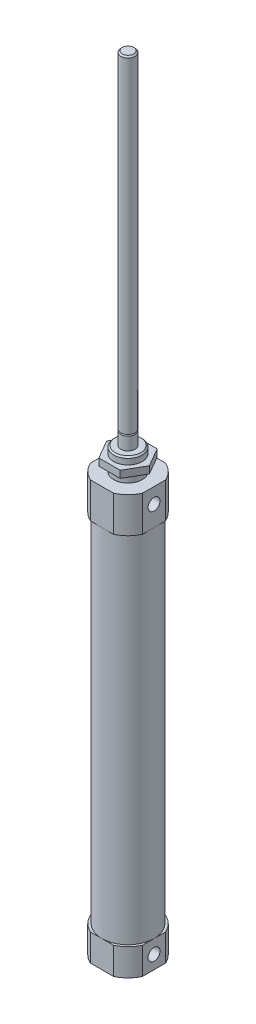
SolidWorks part; units mm, degrees
ref_plane "Front Plane" through (0, 0, 0) normal (0, 0, 1) x (1, 0, 0)
ref_plane "Top Plane" through (0, 0, 0) normal (0, 1, 0) x (1, 0, 0)
ref_plane "Right Plane" through (0, 0, 0) normal (1, 0, 0) x (0, 0, -1)
sketch "Sketch1" plane through (0, 0, 0) normal (0, 1, 0) x (1, 0, 0)
  line L0 (0, 0) -> (0, -50000) construction
  line L1 (-4.0345, 9.15) -> (4.0345, 9.15)
  line L2 (-9.15, 4.0345) -> (-9.15, -4.0345)
  line L3 (-4.0345, -9.15) -> (4.0345, -9.15)
  line L4 (9.15, 4.0345) -> (9.15, -4.0345)
  line L5 (0, 0) -> (50000, 0) construction
  arc A0 (4.0345, -9.15) -> (9.15, -4.0345) centre (0, 0) ccw
  arc A1 (9.15, 4.0345) -> (4.0345, 9.15) centre (0, 0) ccw
  arc A2 (-4.0345, 9.15) -> (-9.15, 4.0345) centre (0, 0) ccw
  arc A3 (-9.15, -4.0345) -> (-4.0345, -9.15) centre (0, 0) ccw
  point P0 (0, 0)
  dimension "D3" = 10
  dimension "D1" = 18.3
  dimension "D2" = 18.3
extrude "Boss-Extrude1" add sketch "Sketch1" along normal blind 12.5
sketch "Sketch3" plane through (0, 0, 0) normal (0, -1, 0) x (1, 0, 0)
  circle A0 centre (0, 0) radius 9.15
  dimension "D1" = 18.3
extrude "Boss-Extrude2" add sketch "Sketch3" along normal blind 125
sketch "Sketch4" plane through (0, -125, 0) normal (0, -1, 0) x (1, 0, 0)
  line L4 (-4.0345, 9.15) -> (4.0345, 9.15)
  line L5 (-9.15, -4.0345) -> (-9.15, 4.0345)
  line L6 (4.0345, -9.15) -> (-4.0345, -9.15)
  line L7 (9.15, 4.0345) -> (9.15, -4.0345)
  arc A4 (-4.0345, 9.15) -> (-9.15, 4.0345) centre (0, 0) ccw
  arc A5 (-9.15, -4.0345) -> (-4.0345, -9.15) centre (0, 0) ccw
  arc A6 (4.0345, -9.15) -> (9.15, -4.0345) centre (0, 0) ccw
  arc A7 (9.15, 4.0345) -> (4.0345, 9.15) centre (0, 0) ccw
extrude "Boss-Extrude3" add sketch "Sketch4" along normal blind 9.5
sketch "Sketch5" plane through (0, 12.5, 0) normal (0, 1, 0) x (1, 0, 0)
  circle A0 centre (0, 0) radius 5
  dimension "D1" = 10
extrude "Boss-Extrude4" add sketch "Sketch5" along normal blind 8
sketch "Sketch6" plane through (0, 20.5, 0) normal (0, 1, 0) x (1, 0, 0)
  circle A0 centre (0, 0) radius 2.5
  dimension "D1" = 5
extrude "Boss-Extrude5" add sketch "Sketch6" along normal blind 5
chamfer "Chamfer1" distance 0.5 angle 45 1 edges at (0, 25.5, 2.5)
sketch "Sketch8" plane through (0, 25.5, 0) normal (0, 1, 0) x (1, 0, 0)
  circle A0 centre (0, 0) radius 2.5
  dimension "D1" = 5
extrude "Boss-Extrude6" add sketch "Sketch8" along normal blind 115
chamfer "Chamfer2" distance 0.5 angle 45 1 edges at (0, 20.5, 5)
ref_plane "Plane1" through (0, 15.5, 0) normal (0, 1, 0) x (1, 0, 0)
sketch "Sketch9" plane through (0, 15.5, 0) normal (0, 1, 0) x (1, 0, 0)
  line L1 (7.5056, 0) -> (3.7528, 6.5)
  line L2 (3.7528, 6.5) -> (-3.7528, 6.5)
  line L3 (-3.7528, 6.5) -> (-7.5056, 0)
  line L4 (-7.5056, 0) -> (-3.7528, -6.5)
  line L5 (-3.7528, -6.5) -> (3.7528, -6.5)
  line L6 (3.7528, -6.5) -> (7.5056, 0)
  circle A0 centre (0, 0) radius 6.5 construction
  dimension "D1" = 13
extrude "Boss-Extrude7" add sketch "Sketch9" along normal blind 2.5
chamfer "Chamfer4" distance 0.5 angle 45 1 edges at (0, 140.5, 2.5)
hole_wizard "M5 Tapped Hole1" positions "Sketch11" profile "Sketch10" tap size "M5" standard "Gb"
sketch "Sketch11" plane through (9.15, 0, 0) normal (1, 0, 0) x (0, 0, -1)
  point P0 (0, 7.1092)
  point P2 (0, -129.8042)
sketch "Sketch10" plane through (9.15, 7.1092, 0) normal (0, 1, 0) x (0, 0, -1)
  line L0 (0, 0) -> (0, 15.2618)
  line L1 (0, 15.2618) -> (2.1, 14)
  line L2 (2.1, 14) -> (2.1, 0)
  line L5 (2.1, 0) -> (0, 0)
  line L10 (0, 15.2618) -> (-2.1, 14) construction
  line L11 (0, -6.35) -> (0, 107.95) construction
  dimension "螺纹孔钻头直径" = 4.2
  dimension "螺纹孔钻头深度" = 14
  dimension "导头角度" = 118
cosmetic thread "Cosmetic thread 1" parameters "D1"=10, "D2"=5
cosmetic thread "Cosmetic thread 2" parameters "D1"=10, "D2"=5
